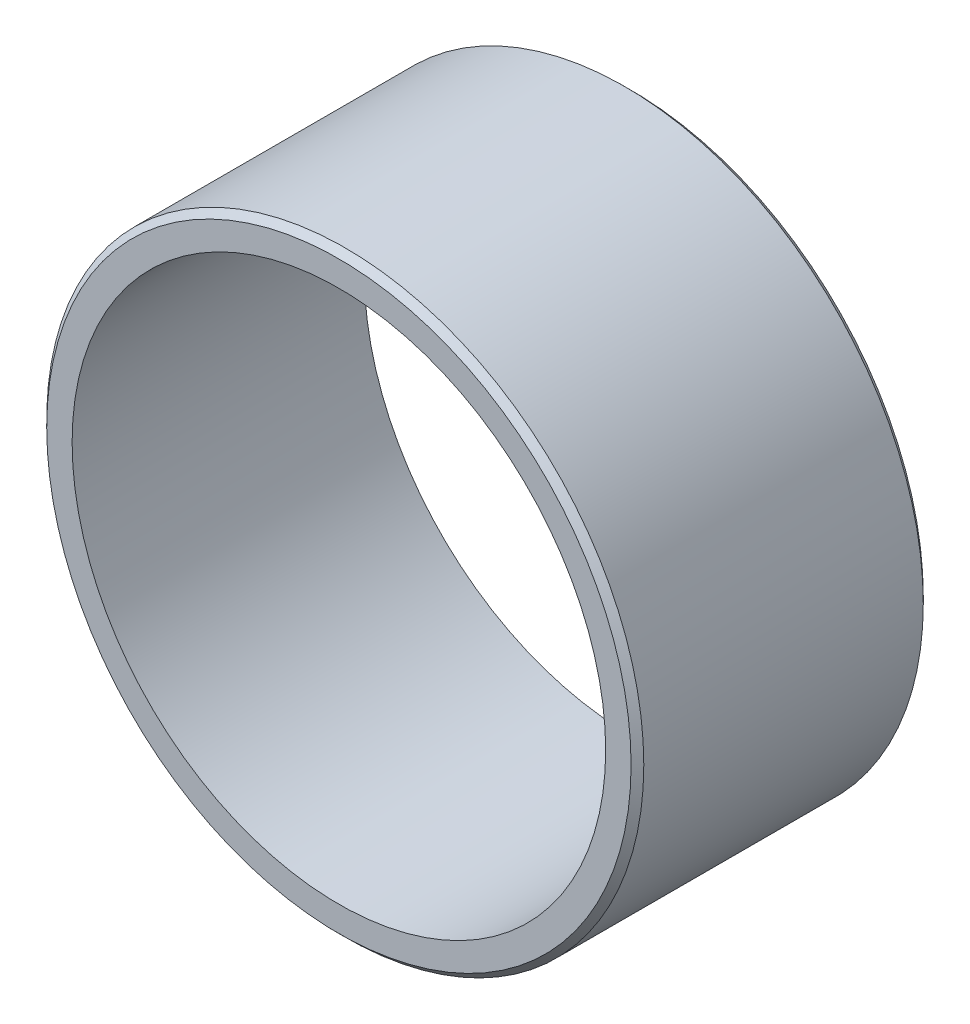
from build123d import *

# Parameters (mm, degrees)
SKETCH1_R           = 23.5
SKETCH1_R_2         = 21
BOSS_EXTRUDE1_DEPTH = 23
CHAMFER1_SIZE       = 0.5


with BuildPart() as part:
    # Sketch1 → Boss-Extrude1 (new body)
    with BuildSketch(Plane.XY):
        Circle(SKETCH1_R)
        Circle(SKETCH1_R_2, mode=Mode.SUBTRACT)
    extrude(amount=BOSS_EXTRUDE1_DEPTH)

    # Chamfer1
    chamfer1_edges = [part.edges().sort_by_distance(p)[0] for p in [
        (-23.5, 0, 0),
        (-23.5, 0, 23),
    ]]
    chamfer(chamfer1_edges, length=CHAMFER1_SIZE)


solid = part.part
